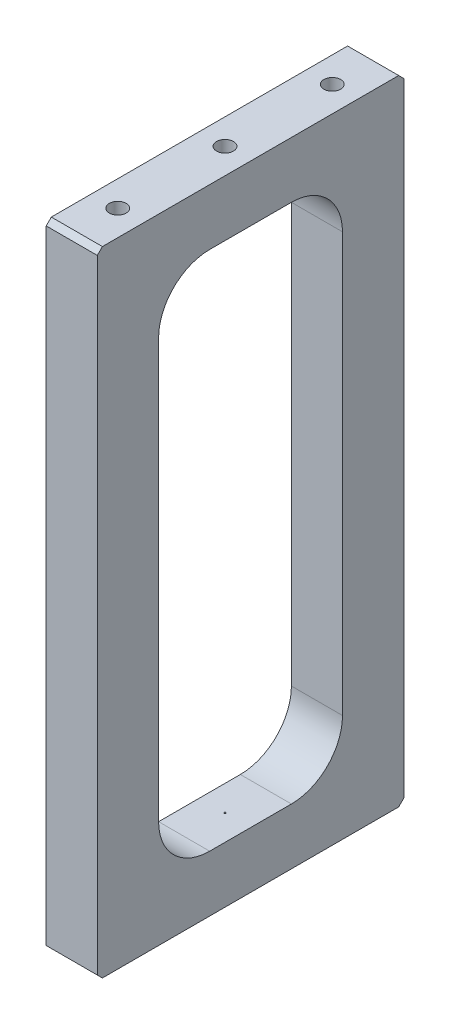
SolidWorks part; units mm, degrees
ref_plane "Front Plane" through (0, 0, 0) normal (0, 0, 1) x (1, 0, 0)
ref_plane "Top Plane" through (0, 0, 0) normal (0, 1, 0) x (1, 0, 0)
ref_plane "Right Plane" through (0, 0, 0) normal (1, 0, 0) x (0, 0, -1)
sketch "Sketch1" plane through (0, 0, 0) normal (1, 0, 0) x (0, 0, -1)
  line L1 (-30, 62) -> (30, 62)
  line L2 (-30, 62) -> (-30, -62)
  line L3 (-30, -62) -> (30, -62)
  line L4 (30, 62) -> (30, -62)
  line L5 (-30, 62) -> (30, -62) construction
  line L6 (-30, -62) -> (30, 62) construction
  point P0 (0, 0)
  dimension "D1" = 124
  dimension "D2" = 60
extrude "Boss-Extrude1" add sketch "Sketch1" along normal mid plane 10
sketch "Sketch2" plane through (5, 0, 0) normal (1, 0, 0) x (0, 0, -1)
  line L1 (-18, 51) -> (18, 51)
  line L2 (-18, 51) -> (-18, -51)
  line L3 (-18, -51) -> (18, -51)
  line L4 (18, 51) -> (18, -51)
  line L5 (-18, 51) -> (18, -51) construction
  line L6 (-18, -51) -> (18, 51) construction
  point P0 (0, 0)
  dimension "D1" = 102
  dimension "D2" = 36
extrude "Cut-Extrude1" cut sketch "Sketch2" against normal through all
hole_wizard "M4 Tapped Hole1" positions "Sketch3" profile "Sketch4" tap size "M4" standard "ISO"
sketch "Sketch3" plane through (0, 62, 0) normal (0, 1, 0) x (1, 0, 0)
  line L0 (0, 0) -> (15.8831, 0) construction
  point P0 (0, 0)
  point P3 (0, 21)
  point P5 (0, -21)
  dimension "D1" = 42
sketch "Sketch4" plane through (0, 62, 0) normal (1, 0, 0) x (0, 0, 1)
  line L0 (0, 0) -> (0, 11.0914)
  line L1 (0, 11.0914) -> (1.65, 10.1)
  line L2 (1.65, 10.1) -> (1.65, 0)
  line L5 (1.65, 0) -> (0, 0)
  line L10 (0, 11.0914) -> (-1.65, 10.1) construction
  line L11 (0, -6.35) -> (0, 107.95) construction
  dimension "螺纹孔钻头直径" = 3.3
  dimension "螺纹孔钻头深度" = 10.1
  dimension "导头角度" = 118
cosmetic thread "Cosmetic Thread1" parameters "D1"=8, "D2"=4
cosmetic thread "Cosmetic Thread2" parameters "D1"=8, "D2"=4
cosmetic thread "Cosmetic Thread3" parameters "D1"=8, "D2"=4
fillet "Fillet1" radius 10 4 edges at (0, -51, 18) (0, -51, -18) (0, 51, -18) (0, 51, 18)
hole_wizard "M4 Tapped Hole2" positions "Sketch5" profile "Sketch6" tap size "M4" standard "ISO"
sketch "Sketch5" plane through (0, -62, 0) normal (0, -1, 0) x (-1, 0, 0)
  line L0 (0, 0) -> (19.6725, 0) construction
  point P0 (0, 0)
  point P3 (0, 21)
  point P5 (0, -21)
  dimension "D1" = 42
sketch "Sketch6" plane through (0, -62, 0) normal (1, 0, 0) x (0, 0, -1)
  line L0 (0, 0) -> (0, 11.0914)
  line L1 (0, 11.0914) -> (1.65, 10.1)
  line L2 (1.65, 10.1) -> (1.65, 0)
  line L5 (1.65, 0) -> (0, 0)
  line L10 (0, 11.0914) -> (-1.65, 10.1) construction
  line L11 (0, -6.35) -> (0, 107.95) construction
  dimension "螺纹孔钻头直径" = 3.3
  dimension "螺纹孔钻头深度" = 10.1
  dimension "导头角度" = 118
cosmetic thread "Cosmetic Thread4" parameters "D1"=8, "D2"=4
cosmetic thread "Cosmetic Thread5" parameters "D1"=8, "D2"=4
cosmetic thread "Cosmetic Thread6" parameters "D1"=8, "D2"=4
chamfer "Chamfer1" distance 1 angle 45 4 edges at (0, -62, -30) (0, -62, 30) (0, 62, -30) (0, 62, 30)
